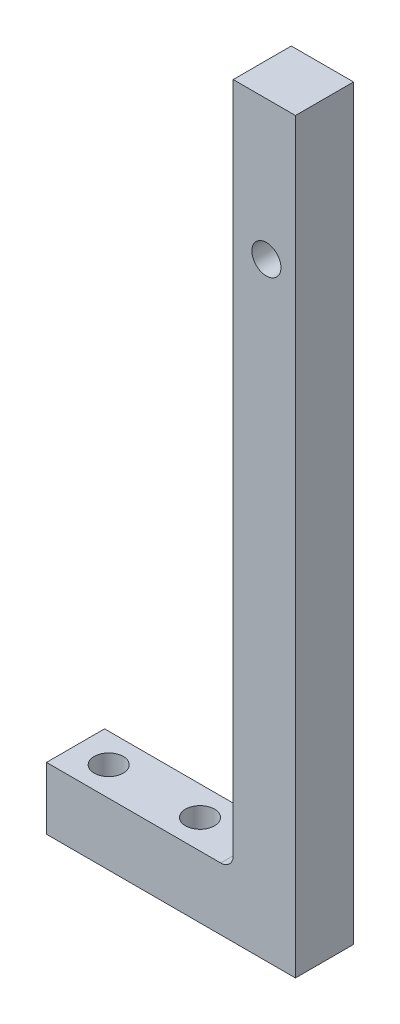
SolidWorks part; units mm, degrees
ref_plane "前视基准面" through (0, 0, 0) normal (0, 0, 1) x (1, 0, 0)
ref_plane "上视基准面" through (0, 0, 0) normal (0, 1, 0) x (1, 0, 0)
ref_plane "右视基准面" through (0, 0, 0) normal (1, 0, 0) x (0, 0, -1)
sketch "草图1" plane through (0, 0, 0) normal (0, 0, 1) x (1, 0, 0)
  line L0 (0, 180) -> (-15, 180)
  line L1 (-15, 180) -> (-15, 15)
  line L2 (-15, 15) -> (-60, 15)
  line L3 (-60, 15) -> (-60, 0)
  line L5 (0, 180) -> (0, 0)
  line L8 (0, 0) -> (-60, 0)
  dimension "D1" = 15
  dimension "D2" = 15
  dimension "D3" = 60
  dimension "D4" = 180
extrude "凸台-拉伸1" add sketch "草图1" along normal mid plane 14
fillet "圆角1" radius 3
sketch "草图3" plane through (0, 15, 0) normal (0, 1, 0) x (1, 0, 0)
  line L0 (-60, -7) -> (-60, 7) construction
  circle A0 centre (-52, 0) radius 3.5
  circle A1 centre (-30, 0) radius 3.5
  dimension "D1" = 7
  dimension "D2" = 22
  dimension "D3" = 8
extrude "切除-拉伸1" cut sketch "草图3" against normal up to next
sketch "草图4" plane through (0, 0, -7) normal (0, 0, -1) x (-1, 0, 0)
  circle A0 centre (7, 146.5) radius 3.5
  dimension "D1" = 7
extrude "切除-拉伸2" cut sketch "草图4" against normal up to next
